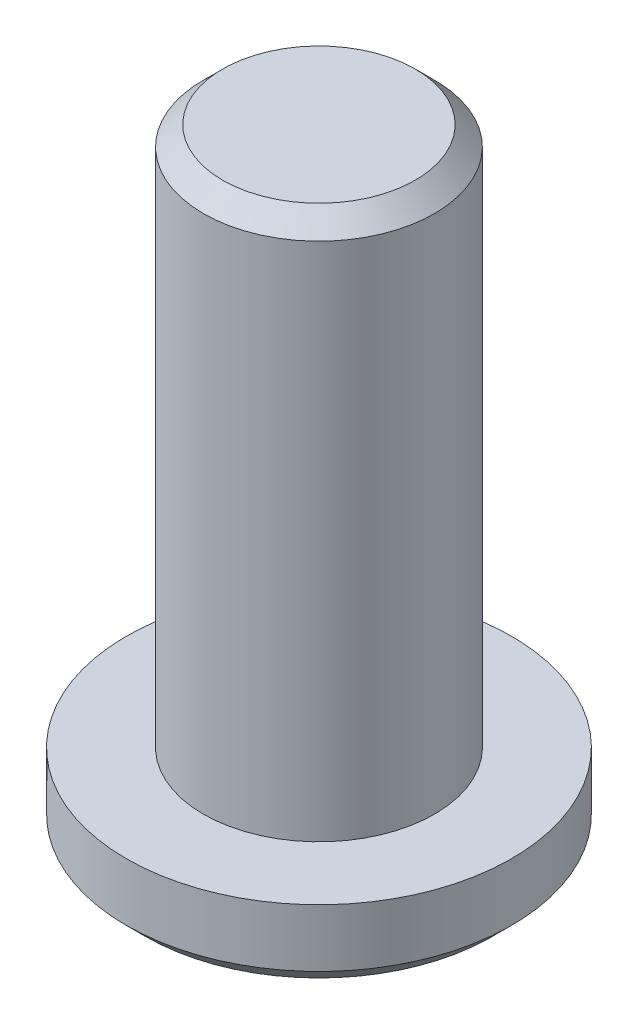
SolidWorks part; units mm, degrees
ref_plane "Front Plane" through (0, 0, 0) normal (0, 0, 1) x (1, 0, 0)
ref_plane "Top Plane" through (0, 0, 0) normal (0, 1, 0) x (1, 0, 0)
ref_plane "Right Plane" through (0, 0, 0) normal (1, 0, 0) x (0, 0, -1)
sketch "Sketch1" plane through (0, 0, 0) normal (0, 1, 0) x (1, 0, 0)
  circle A0 centre (0, 0) radius 5
  dimension "D1" = 10
extrude "Boss-Extrude1" add sketch "Sketch1" along normal blind 2
sketch "Sketch2" plane through (0, 2, 0) normal (0, 1, 0) x (1, 0, 0)
  circle A0 centre (0, 0) radius 3
  dimension "D1" = 6
extrude "Boss-Extrude2" add sketch "Sketch2" along normal blind 14
chamfer "Chamfer1" distance 0.5 angle 45 2 edges at (0, 16, 3) (0, 0, 5)
